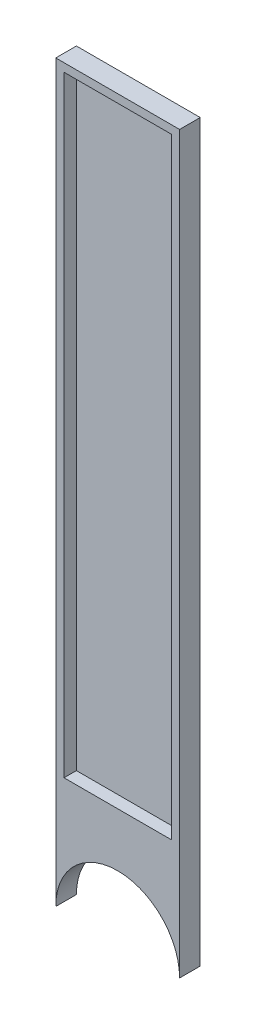
SolidWorks part; units mm, degrees
ref_plane "Front Plane" through (0, 0, 0) normal (0, 0, 1) x (1, 0, 0)
ref_plane "Top Plane" through (0, 0, 0) normal (0, 1, 0) x (1, 0, 0)
ref_plane "Right Plane" through (0, 0, 0) normal (1, 0, 0) x (0, 0, -1)
other "Configuration Table"
sketch "Sketch1" plane through (0, 0, 0) normal (0, 0, 1) x (1, 0, 0)
  line L1 (30, 178) -> (0, 178)
  line L2 (30, 178) -> (30, 0)
  line L3 (30, 0) -> (0, 0)
  line L4 (0, 178) -> (0, 0)
  dimension "D1" = 30
  dimension "D2" = 178
extrude "Boss-Extrude1" add sketch "Sketch1" along normal blind 5
sketch "Sketch3" plane through (0, 0, 5) normal (0, 0, 1) x (1, 0, 0)
  line L0 (0, 178) -> (0, 0) construction
  line L1 (2, 176) -> (28, 176)
  line L2 (2, 176) -> (2, -34)
  line L3 (2, -34) -> (28, -34)
  line L4 (28, 176) -> (28, -34)
  line L6 (30, 0) -> (30, 178) construction
  line L7 (30, 178) -> (0, 178) construction
  dimension "D1" = 2
  dimension "D2" = 2
  dimension "D3" = 2
  dimension "D4" = 210
extrude "Cut-Extrude1" cut sketch "Sketch3" against normal blind 3
sketch "Sketch4" plane through (0, 0, 2) normal (0, 0, 1) x (1, 0, 0)
  line L0 (2, 28) -> (28, 28)
  line L1 (2, 176) -> (2, 0) construction
  line L2 (28, 0) -> (28, 176) construction
  line L3 (28, 28) -> (28, 18)
  line L4 (28, 18) -> (2, 18)
  line L5 (2, 18) -> (2, 28)
  line L6 (28, 176) -> (2, 176) construction
  dimension "D1" = 148
  dimension "D2" = 10
extrude "Boss-Extrude2" add sketch "Sketch4" along normal up to surface (3 mm away) contours L4 L5 L0 L3 up to face at (15, 88.5, 5)
sketch "Sketch5" plane through (0, 0, 2) normal (0, 0, 1) x (1, 0, 0)
  line L0 (15, 18) -> (15, 0) construction
  line L1 (28, 18) -> (2, 18) construction
  line L2 (2, 0) -> (28, 0) construction
  line L3 (0, 0) -> (30, 0)
  arc A0 (0, 0) -> (30, 0) centre (15, 0) cw
  dimension "D1" = 15
extrude "Cut-Extrude3" cut sketch "Sketch5" along normal mid plane 10 contours L3 A0
sketch "Sketch6" plane through (0, 0, 2) normal (0, 0, 1) x (1, 0, 0)
  line L6 (28, 7.4833) -> (28, 18)
  line L7 (28, 18) -> (2, 18)
  line L8 (2, 18) -> (2, 7.4833)
  line L9 (28, 7.4833) -> (28, 18)
  line L10 (28, 18) -> (2, 18)
  line L11 (2, 18) -> (2, 7.4833)
  arc A2 (28, 7.4833) -> (2, 7.4833) centre (15, 0) ccw
  arc A3 (28, 7.4833) -> (2, 7.4833) centre (15, 0) ccw
  dimension "D1" = 0
extrude "Boss-Extrude3" add sketch "Sketch6" along normal up to surface (3 mm away) up to face at (15, 50.9037, 5)
